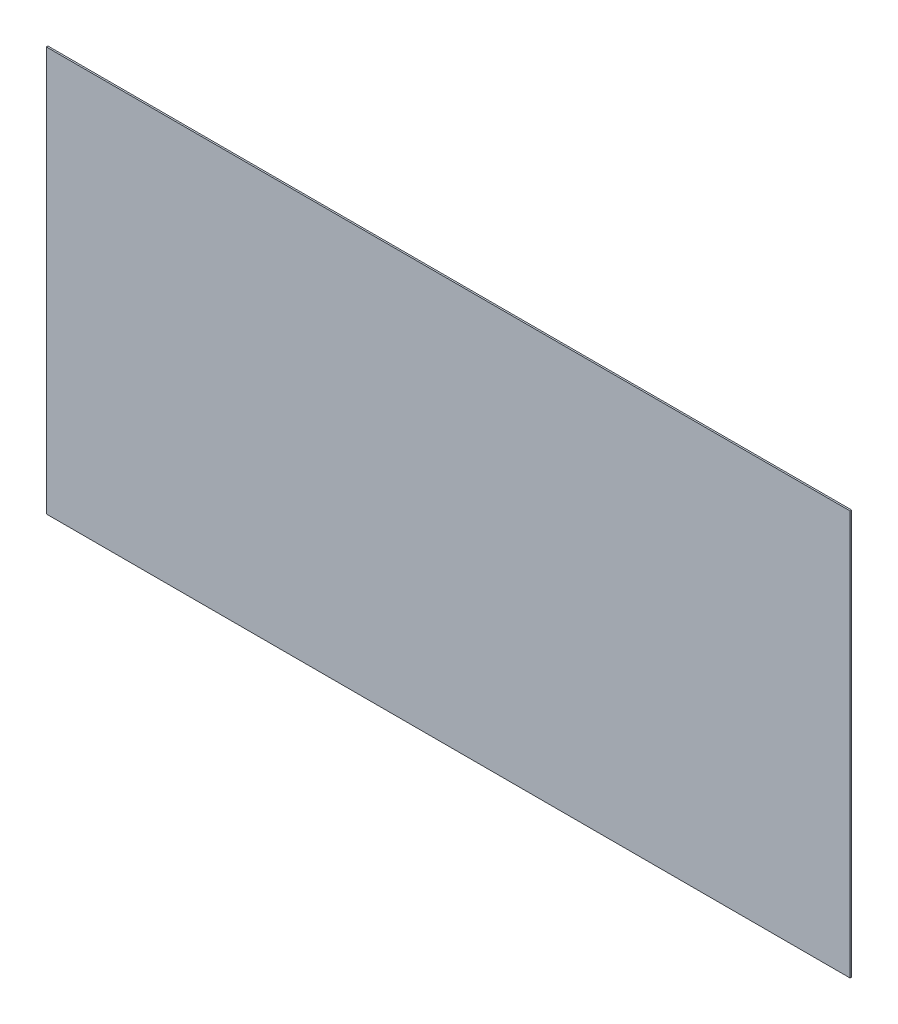
SolidWorks part; units mm, degrees
material "普通碳钢"
ref_plane "Front Plane" through (0, 0, 0) normal (0, 0, 1) x (1, 0, 0)
ref_plane "Top Plane" through (0, 0, 0) normal (0, 1, 0) x (1, 0, 0)
ref_plane "Right Plane" through (0, 0, 0) normal (1, 0, 0) x (0, 0, -1)
sketch "Sketch1" plane through (0, 0, 0) normal (0, 0, 1) x (1, 0, 0)
  line L5 (0, 0) -> (3000, 0)
  line L6 (0, 0) -> (0, 1510)
  line L7 (0, 1510) -> (3000, 1510)
  line L8 (3000, 0) -> (3000, 1510)
  dimension "D2" = 1510
  dimension "D3" = 3000
extrude "Boss-Extrude1" add sketch "Sketch1" along normal blind 6
